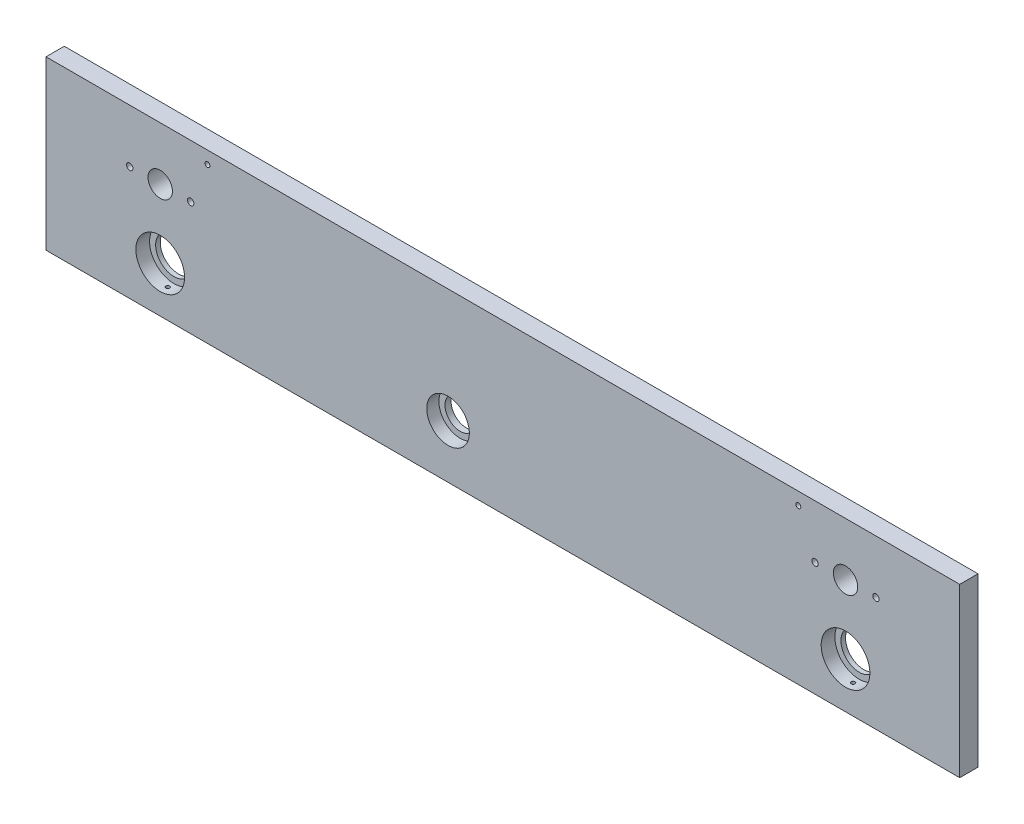
from build123d import *

# Parameters (mm, degrees)
EXTRUDE_1_DEPTH         = 12
SKETCH_2_R              = 16
CUT_EXTRUDE_2_DEPTH     = 9
SKETCH_3_R              = 14
CUT_EXTRUDE_3_DEPTH     = 8
SKETCH_4_R              = 10
CUT_EXTRUDE_4_DEPTH     = 320.631037291
HOLE_WIZARD_M4_2_D      = 3.3
HOLE_WIZARD_M4_3_D      = 3.3
HOLE_WIZARD_M4_3_DEPTH  = 12.1
HOLE_WIZARD_M4_3_TIP    = 0.991420021
HOLE_WIZARD_M3_1_REACH  = 321.756
HOLE_WIZARD_M3_1_BORE_R = 1.25
SKETCH_17_R             = 12
CUT_EXTRUDE_5_DEPTH     = 320.657629385
SKETCH_18_R             = 8
CUT_EXTRUDE_6_DEPTH     = 320.756157129
HOLE_WIZARD_M5_1_D      = 4.2


with BuildPart() as part:
    # 草图1 → 凸台-拉伸1 (new body)
    with BuildSketch(Plane.XY):
        Polygon((-300, -30), (-300, 0), (300, 0), (300, -30), (300, -110), (-300, -110), align=None)
    extrude(amount=EXTRUDE_1_DEPTH)

    # 草图2 → 切除-拉伸2 (cut)
    with BuildSketch(Plane.XY.offset(12)):
        with Locations(Location((225, -80, 0), (0, 0, 180))):
            Circle(SKETCH_2_R)
        with Locations((-225, -80)):
            Circle(SKETCH_2_R)
    extrude(amount=-CUT_EXTRUDE_2_DEPTH, mode=Mode.SUBTRACT)

    # 草图3 → 切除-拉伸3 (cut)
    with BuildSketch(Plane.XY.offset(12)):
        with Locations((-36, -75)):
            Circle(SKETCH_3_R)
    extrude(amount=-CUT_EXTRUDE_3_DEPTH, mode=Mode.SUBTRACT)

    # 草图4 → 切除-拉伸4 (cut, through all)
    with BuildSketch(Plane.XY.offset(4)):
        with Locations((-36, -75)):
            Circle(SKETCH_4_R)
    extrude(amount=-CUT_EXTRUDE_4_DEPTH, mode=Mode.SUBTRACT)

    # M4 螺纹孔2 (through all)
    with Locations(Plane(origin=(0, 0, 0), x_dir=(-1, 0, 0), z_dir=(0, 0, -1))):
        with Locations((-194, -8.25), (194, -8.25)):
            Hole(HOLE_WIZARD_M4_2_D / 2)

    # M4 螺纹孔3
    with Locations(Plane(origin=(0, -110, 0), x_dir=(-1, 0, 0), z_dir=(0, -1, 0))):
        with Locations((-262, -6), (-92, -6), (92, -6), (262, -6)):
            Hole(HOLE_WIZARD_M4_3_D / 2, depth=HOLE_WIZARD_M4_3_DEPTH)
            with Locations((0, 0, -(HOLE_WIZARD_M4_3_DEPTH + HOLE_WIZARD_M4_3_TIP / 2))):  # 118° drill point
                Cone(0, HOLE_WIZARD_M4_3_D / 2, HOLE_WIZARD_M4_3_TIP, mode=Mode.SUBTRACT)

    # M3 螺纹孔1 bore → M3 螺纹孔1 (cut, up to next)
    with BuildSketch(Plane(origin=(0, -110, 0), x_dir=(-1, 0, 0), z_dir=(0, -1, 0)), mode=Mode.PRIVATE) as hole_wizard_m3_1_sk1:
        with Locations((225, -7)):
            Circle(HOLE_WIZARD_M3_1_BORE_R)
    hole_wizard_m3_1_tool1 = extrude(hole_wizard_m3_1_sk1.sketch, amount=-HOLE_WIZARD_M3_1_REACH, mode=Mode.PRIVATE) & part.part
    # M3 螺纹孔1 bore → M3 螺纹孔1 (cut, up to next)
    with BuildSketch(Plane(origin=(0, -110, 0), x_dir=(-1, 0, 0), z_dir=(0, -1, 0)), mode=Mode.PRIVATE) as hole_wizard_m3_1_sk2:
        with Locations((-225, -7)):
            Circle(HOLE_WIZARD_M3_1_BORE_R)
    hole_wizard_m3_1_tool2 = extrude(hole_wizard_m3_1_sk2.sketch, amount=-HOLE_WIZARD_M3_1_REACH, mode=Mode.PRIVATE) & part.part
    add(hole_wizard_m3_1_tool1.solids().sort_by_distance((-225, -110, 7))[0], mode=Mode.SUBTRACT)
    add(hole_wizard_m3_1_tool2.solids().sort_by_distance((225, -110, 7))[0], mode=Mode.SUBTRACT)

    # 草图17 → 切除-拉伸5 (cut, through all)
    with BuildSketch(Plane.XY.offset(3)):
        with Locations((-225, -80)):
            Circle(SKETCH_17_R)
        with Locations((225, -80)):
            Circle(SKETCH_17_R)
    extrude(amount=-CUT_EXTRUDE_5_DEPTH, mode=Mode.SUBTRACT)

    # 草图18 → 切除-拉伸6 (cut, through all)
    with BuildSketch(Plane.XY.offset(12)):
        with Locations((-225, -35)):
            Circle(SKETCH_18_R)
        with Locations((225, -35)):
            Circle(SKETCH_18_R)
    extrude(amount=-CUT_EXTRUDE_6_DEPTH, mode=Mode.SUBTRACT)

    # M5 螺纹孔1 (through all)
    with Locations(Plane.XY.offset(12)):
        with Locations((245, -35), (205, -35), (-245, -35), (-205, -35)):
            Hole(HOLE_WIZARD_M5_1_D / 2)


solid = part.part
